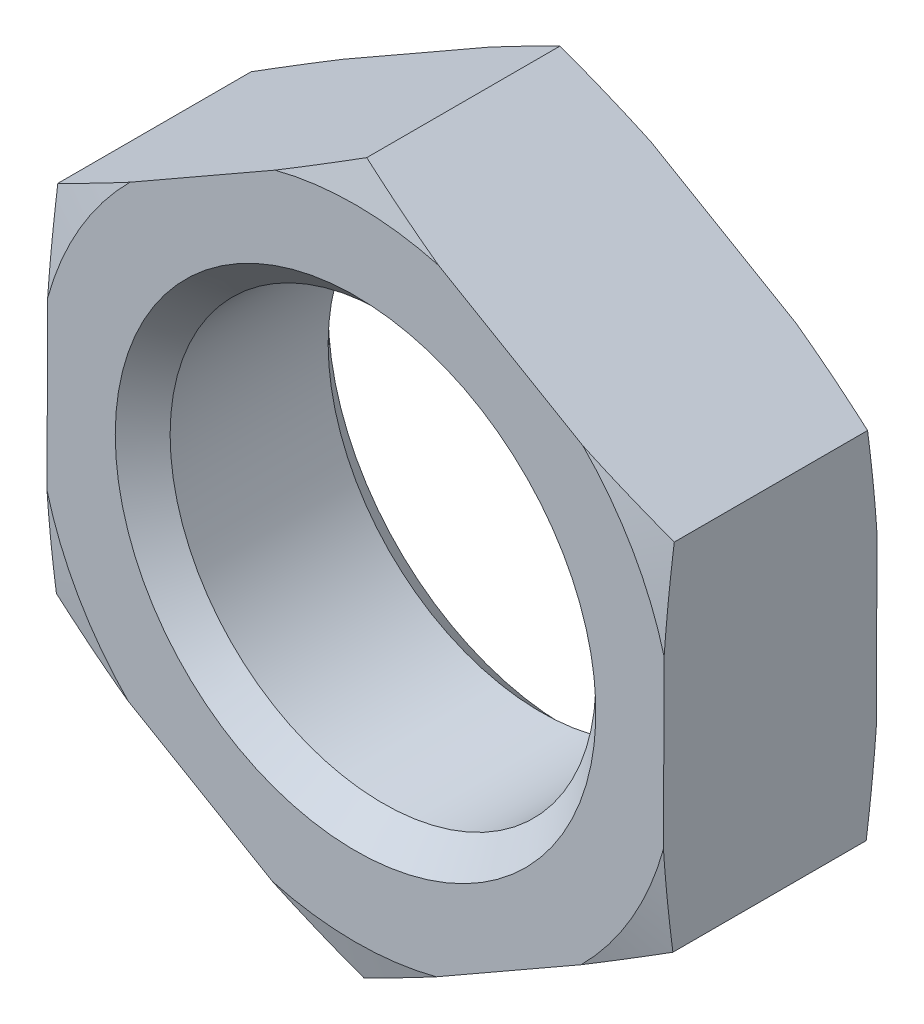
SolidWorks part; units mm, degrees
extrude "Base-Extrude" add sketch "Sketch1" along normal blind 8
sketch "Sketch1" plane through (0, 0, 0) normal (0, 0, 1) x (1, 0, 0)
  line L0 (-26.8088, 0) -> (37.1748, 0) construction
  line L1 (0, 25.0215) -> (0, -25.0215) construction
  line L3 (0.0526, 13.3749) -> (-11.5567, 6.733)
  line L4 (-11.5567, 6.733) -> (-11.6093, -6.6419)
  line L5 (-11.6093, -6.6419) -> (-0.0526, -13.3749)
  line L6 (-0.0526, -13.3749) -> (11.5567, -6.733)
  line L7 (11.5567, -6.733) -> (11.6093, 6.6419)
  line L8 (11.6093, 6.6419) -> (0.0526, 13.3749)
  circle A0 centre (0, 0) radius 11.5831 construction
  circle A1 centre (0, 0) radius 8
cosmetic thread "Cosmetic Thread1"
chamfer "Chamfer1" distance 1.031 angle 45 2 edges at (8, 0, 0) (8, 0, 8)
ref_plane "Plane1" through (0, 0, 0) normal (0, 0, 1) x (1, 0, 0)
ref_plane "Plane2" through (0, 0, 0) normal (0, 1, 0) x (1, 0, 0)
ref_plane "Plane3" through (0, 0, 0) normal (1, 0, 0) x (0, 0, -1)
sketch "Dimension Sketch" plane through (0, 0, 0) normal (0, 0, 1) x (1, 0, 0)
  line L0 (0, 0) -> (24.1005, 0)
  line L1 (27.4249, 65.7219) -> (44.7249, 65.7219)
  line L2 (46.8781, 65.7219) -> (69.3781, 65.7219)
  line L3 (-37.8187, 0) -> (-22.5806, 0)
  point P3 (16, 0)
  point P4 (1.5, 0)
  point P5 (26.75, 0)
  point P6 (8, 0)
  point P7 (24.32, 0)
  point P8 (24, 0)
sketch "Sketch2" plane through (0, 0, 0) normal (0, 0, -1) x (-1, 0, 0)
  circle A0 centre (0, 0) radius 12
  circle A1 centre (0, 0) radius 8 construction
extrude "Cut-Extrude1" cut sketch "Sketch2" against normal through all draft 75 flip side to cut
sketch "Sketch3" plane through (0, 0, 8) normal (0, 0, 1) x (1, 0, 0)
  circle A0 centre (0, 0) radius 12
extrude "Cut-Extrude2" cut sketch "Sketch3" against normal through all draft 75 flip side to cut
equation "\"e@Sketch1\" = \"e@Dimension Sketch\""
equation "\"D1@Dimension Sketch\" = \"D@Dimension Sketch\" / 1.05"
equation "\"D@Sketch1\" = \"D@Dimension Sketch\""
equation "\"m@Base-Extrude\" = \"m@Dimension Sketch\""
equation "\"D1@Sketch3\" = \"s@Dimension Sketch\""
equation "\"s@Sketch2\" = \"s@Dimension Sketch\""
equation "\"D2@Cosmetic Thread1\" = 1.05 * \"D1@Dimension Sketch\""
equation "\"D1@Chamfer1\" =  ( \"da@Dimension Sketch\" - \"D1@Dimension Sketch\" )  / 2"
